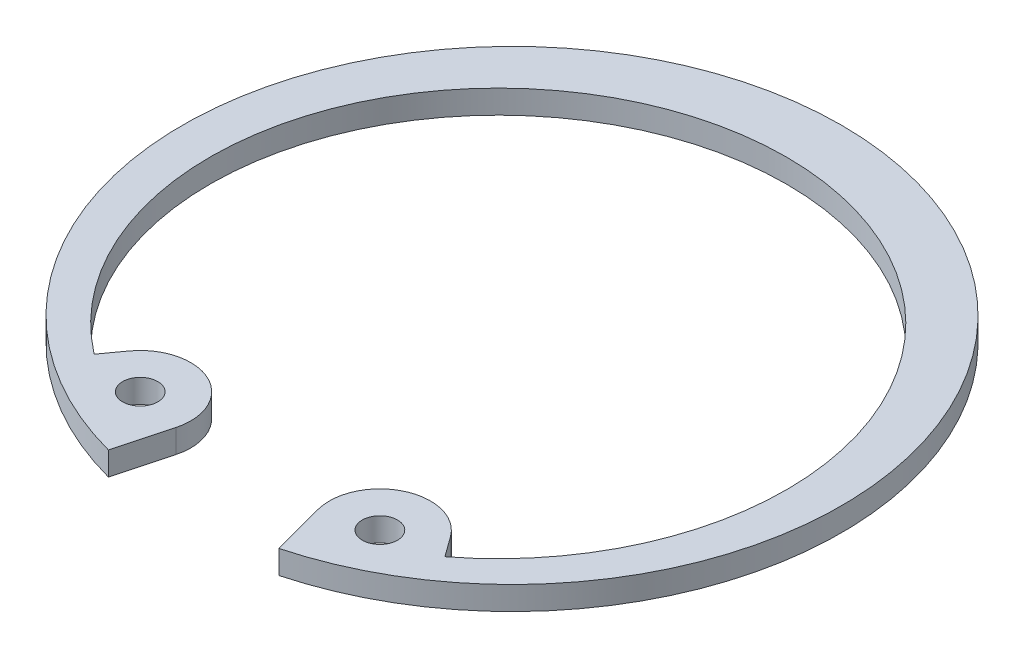
from build123d import *

# Parameters (mm, degrees)
SKETCH2_R           = 1.5
BOSS_EXTRUDE1_DEPTH = 2


with BuildPart() as part:
    # Sketch2 → Boss-Extrude1 (new body)
    with BuildSketch(Plane(origin=(0, 0, 0), x_dir=(1, 0, 0), z_dir=(0, 1, 0))):
        with BuildLine():
            Line((-14.953942403, -20.676544339), (-13.710907235, -18.957822206))
            ThreePointArc((-13.710907235, -18.957822206), (-8.367273859, -17.591450428), (-6.055414365, -22.599114073))
            Line((-6.055414365, -22.599114073), (-7.272815167, -27.142515719))
            ThreePointArc((-7.272815167, -27.142515719), (0, 28.1), (7.272815167, -27.142515719))
            Line((7.272815167, -27.142515719), (6.055414365, -22.599114073))
            ThreePointArc((6.055414365, -22.599114073), (8.367273859, -17.591450428), (13.710907235, -18.957822206))
            Line((13.710907235, -18.957822206), (14.953942403, -20.676544339))
            ThreePointArc((14.953942403, -20.676544339), (0, 23.4), (-14.953942403, -20.676544339))
        make_face()
        with Locations(Location((-10.218554677, -21.483603988, 0), (0, 0, 270))):
            Circle(SKETCH2_R, mode=Mode.SUBTRACT)
        with Locations(Location((10.218554677, -21.483603988, 0), (0, 0, 90))):
            Circle(SKETCH2_R, mode=Mode.SUBTRACT)
    extrude(amount=BOSS_EXTRUDE1_DEPTH)


solid = part.part
